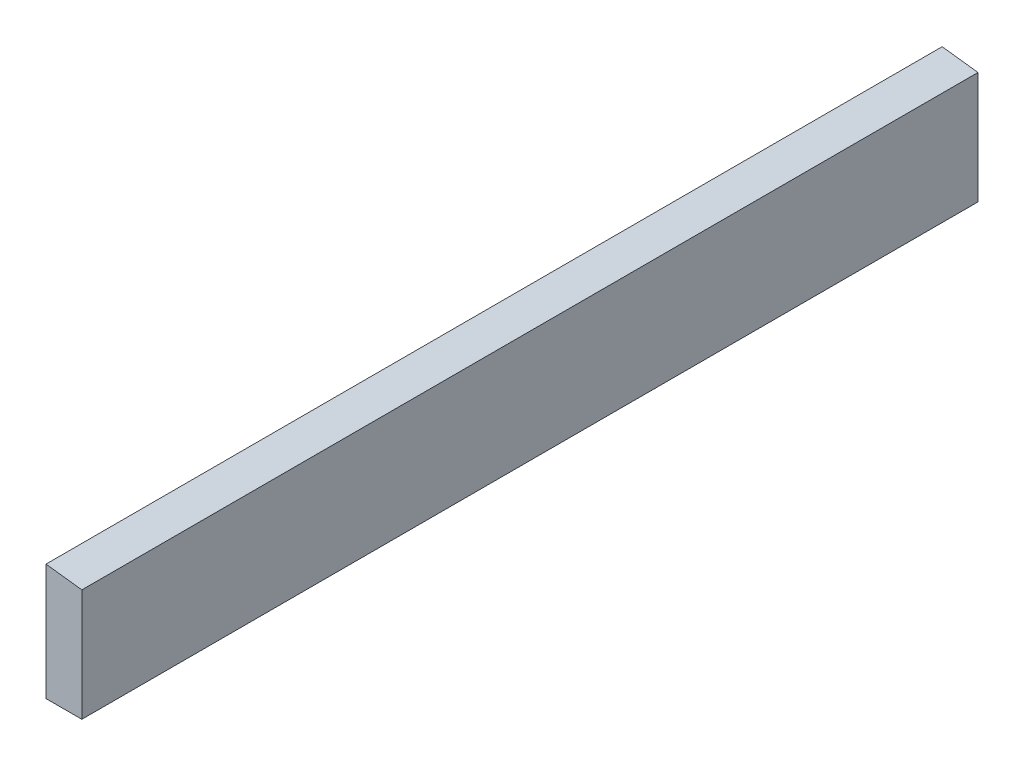
from build123d import *

# Parameters (mm, degrees)
BOSS_EXTRUDE1_DEPTH = 250


with BuildPart() as part:
    # Sketch1 → Boss-Extrude1 (new body)
    with BuildSketch(Plane.XY):
        Polygon((0, 0), (0, 32.5), (10, 31.272154391), (10, 0), align=None)
    extrude(amount=BOSS_EXTRUDE1_DEPTH)


solid = part.part
